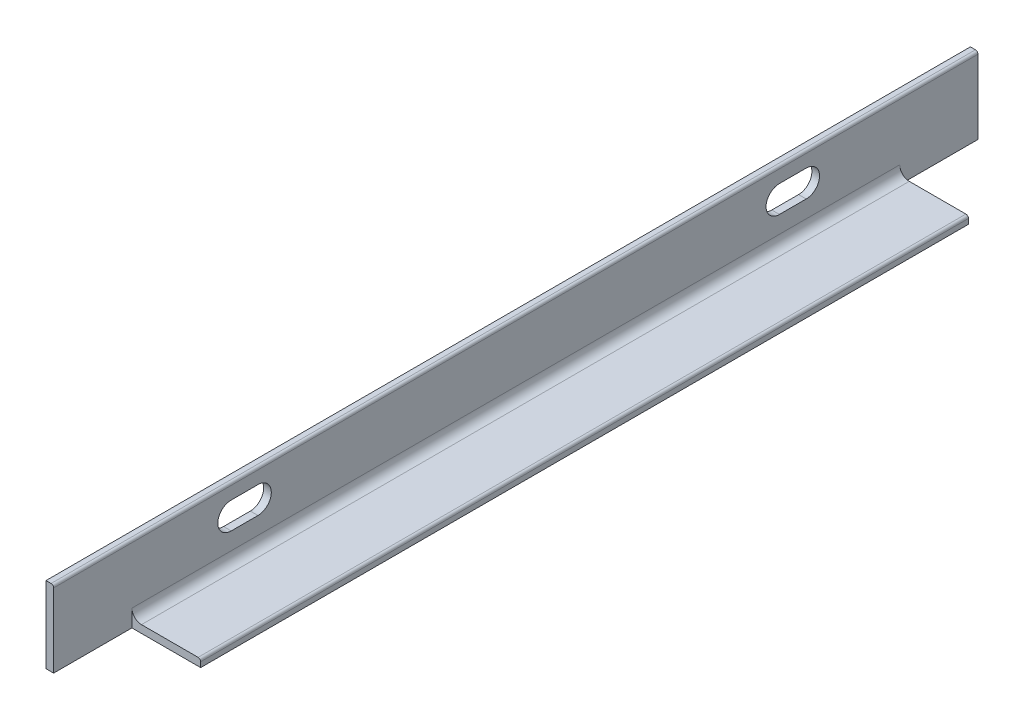
SolidWorks part; units mm, degrees
material "Q235A"
ref_plane "Front Plane" through (0, 0, 0) normal (0, 0, 1) x (1, 0, 0)
ref_plane "Top Plane" through (0, 0, 0) normal (0, 1, 0) x (1, 0, 0)
ref_plane "Right Plane" through (0, 0, 0) normal (1, 0, 0) x (0, 0, -1)
sketch "Sketch1" plane through (0, 0, 0) normal (0, 0, 1) x (1, 0, 0)
  line L0 (0, 0) -> (40, 0)
  line L1 (0, 0) -> (0, 40)
  dimension "D1" = 40
  dimension "D2" = 40
extrude "Extrude-Thin1" add sketch "Sketch1" along normal blind 484.14 thin thin type one direction wall 4
fillet "Fillet1" radius 5 1 edges at (4, 4, 242.07)
fillet "Fillet2" radius 1.3333 2 edges at (40, 4, 242.07) (4, 40, 242.07)
sketch "Sketch2" plane through (0, 0, 0) normal (0, -1, 0) x (1, 0, 0)
  line L0 (0, 484.14) -> (0, 0) construction
  line L1 (40, 0) -> (4, 0)
  line L2 (40, 0) -> (40, 41)
  line L3 (40, 41) -> (4, 41)
  line L4 (4, 0) -> (4, 41)
  dimension "D1" = 4
  dimension "D2" = 41
extrude "Cut-Extrude1" cut sketch "Sketch2" against normal through all
sketch "Sketch3" plane through (0, 0, 0) normal (0, -1, 0) x (1, 0, 0)
  line L0 (40, 484.14) -> (40, 41) construction
  line L1 (40, 484.14) -> (0, 484.14) construction
  line L5 (0, 484.14) -> (0, 0) construction
  line L12 (4, 484.14) -> (40, 484.14)
  line L13 (4, 484.14) -> (4, 443.14)
  line L14 (4, 443.14) -> (40, 443.14)
  line L15 (40, 484.14) -> (40, 443.14)
  dimension "D7" = 4
  dimension "D8" = 41
extrude "Cut-Extrude3" cut sketch "Sketch3" against normal through all
sketch "Sketch4" plane through (4, 0, 0) normal (1, 0, 0) x (0, 0, -1)
  line L0 (-391.14, 25) -> (-377.14, 25) construction
  line L1 (-391.14, 32) -> (-377.14, 32)
  line L2 (-391.14, 18) -> (-377.14, 18)
  line L3 (-484.14, 40) -> (0, 40) construction
  line L5 (-484.14, 0) -> (-484.14, 38.6667) construction
  arc A0 (-391.14, 32) -> (-391.14, 18) centre (-391.14, 25) ccw
  arc A1 (-377.14, 18) -> (-377.14, 32) centre (-377.14, 25) ccw
  point P2 (-384.14, 25)
  point P9 (-484.14, 19.3333)
  dimension "D2" = 7
  dimension "D3" = 100
  dimension "D1" = 15
  dimension "D4" = 14
extrude "Cut-Extrude4" cut sketch "Sketch4" against normal blind 14
pattern_linear "LPattern1" count 2 spacing 287.14 along (0, 0, -1) of "Cut-Extrude4"
